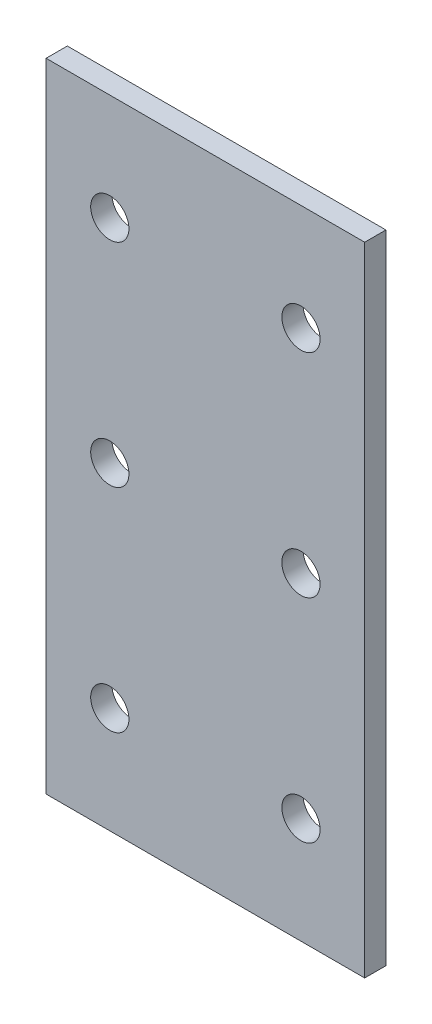
from build123d import *

# Parameters (mm, degrees)
SKETCH1_W           = 150
SKETCH1_H           = 300
SKETCH1_R           = 9
BOSS_EXTRUDE1_DEPTH = 10


with BuildPart() as part:
    # Sketch1 → Boss-Extrude1 (new body)
    with BuildSketch(Plane.XY):
        Rectangle(SKETCH1_W, SKETCH1_H)
        with Locations((-45, 100)):
            Circle(SKETCH1_R, mode=Mode.SUBTRACT)
        with Locations((-45, 0)):
            Circle(SKETCH1_R, mode=Mode.SUBTRACT)
        with Locations((-45, -100)):
            Circle(SKETCH1_R, mode=Mode.SUBTRACT)
        with Locations(Location((45, -100, 0), (0, 0, 180))):
            Circle(SKETCH1_R, mode=Mode.SUBTRACT)
        with Locations(Location((45, 0, 0), (0, 0, 180))):
            Circle(SKETCH1_R, mode=Mode.SUBTRACT)
        with Locations(Location((45, 100, 0), (0, 0, 180))):
            Circle(SKETCH1_R, mode=Mode.SUBTRACT)
    extrude(amount=BOSS_EXTRUDE1_DEPTH)


solid = part.part
